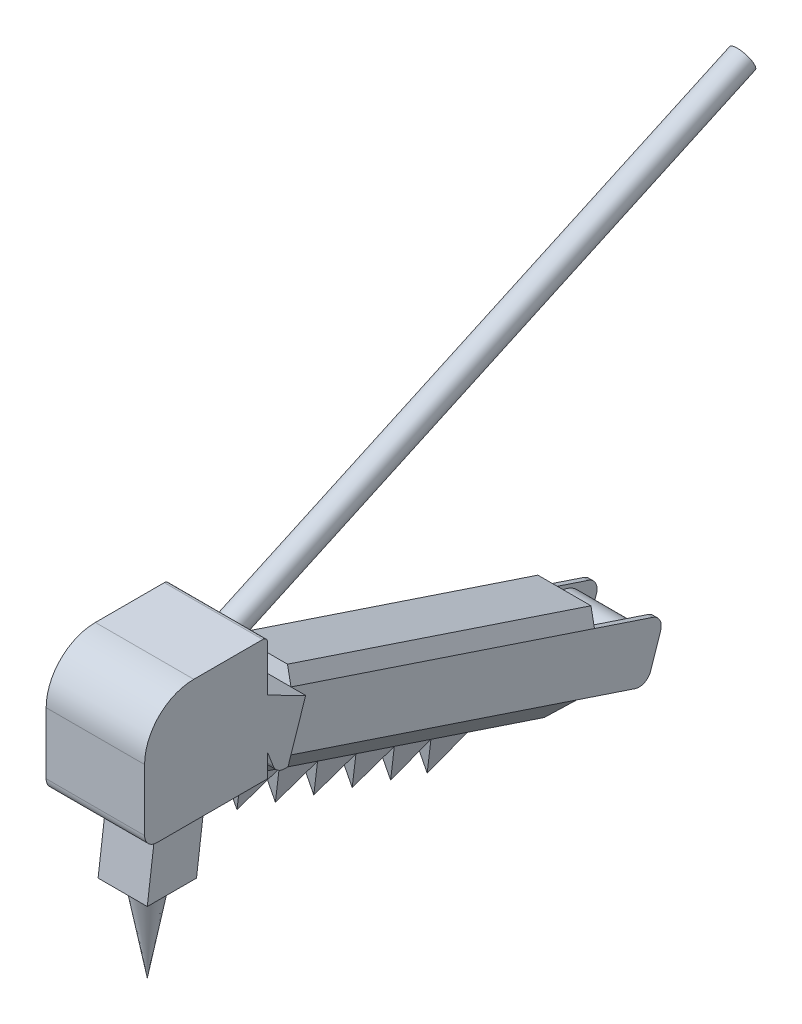
SolidWorks part; units mm, degrees
ref_plane "Front Plane" through (0, 0, 0) normal (0, 0, 1) x (1, 0, 0)
ref_plane "Top Plane" through (0, 0, 0) normal (0, 1, 0) x (1, 0, 0)
ref_plane "Right Plane" through (0, 0, 0) normal (1, 0, 0) x (0, 0, -1)
other "Configuration Table"
sketch "Sketch2" plane through (0, 0, 0) normal (1, 0, 0) x (0, 0, -1)
  line L8 (0, 0) -> (0, 50)
  line L9 (0, 50) -> (50, 50)
  line L10 (50, 50) -> (50, 29.4102)
  line L16 (50, 0) -> (0, 0)
  line L17 (50, 0) -> (50, 9.232)
  line L22 (50, 9.232) -> (53.5278, 0.0614)
  line L25 (65.4524, 21.5893) -> (50, 29.4102)
  line L26 (53.5278, 0.0614) -> (58.2765, 0.0614)
  line L27 (65.4524, 21.5893) -> (58.2765, 0.0614)
  dimension "D1" = 50
  dimension "D2" = 50
  dimension "D3" = 50
extrude "Boss-Extrude1" add sketch "Sketch2" along normal blind 40
fillet "Fillet1" radius 20 1 edges at (20, 50, 0)
fillet "Fillet2" radius 5 1 edges at (20, 0, 0)
ref_plane "Plane1" through (20, 0, 0) normal (1, 0, 0) x (0, 0, -1)
sketch "Sketch4" plane through (20, 0, 0) normal (1, 0, 0) x (0, 0, -1)
  line L0 (25, 6.5797) -> (25, -21.4147) construction
  line L1 (15, 0) -> (11.0974, -30.529)
  line L2 (5, 0) -> (50, 0) construction
  line L3 (11.0974, -30.529) -> (31.0974, -30.529)
  line L4 (31.0974, -30.529) -> (35, 0)
  line L5 (0, 30) -> (0, 5) construction
  line L6 (50, 0) -> (50, 9.232) construction
  line L7 (15, 0) -> (35, 0)
  dimension "D1" = 15
  dimension "D2" = 15
  dimension "D3" = 10
extrude "Boss-Extrude2" add sketch "Sketch4" along normal mid plane 20
sketch "Sketch5" plane through (20, 0, 0) normal (1, 0, 0) x (0, 0, -1)
  line L0 (21.0974, -30.529) -> (21.0974, -46.9338) construction
  line L1 (11.0974, -30.529) -> (31.0974, -30.529) construction
  line L2 (21.0974, -30.529) -> (27.6649, -30.529)
  line L3 (27.6649, -30.529) -> (21.0974, -65.6782)
  line L4 (21.0974, -30.529) -> (21.0974, -65.6782)
revolve "Revolve1" add sketch "Sketch5" angle 360 about L0
fillet "Fillet3" radius 5 1 edges at (20, 0.0614, -53.5278)
fillet "Fillet4" radius 2 1 edges at (20, 50, -50)
sketch "Sketch7" plane through (0, -17.4768, -52.4304) normal (0, -0.3162, -0.9487) x (-1, 0, 0)
  line L1 (-5.963, 18.4869) -> (-16, 8.3482)
  line L2 (-34.037, 18.4869) -> (-24, 8.3482)
  line L5 (-24, 8.3482) -> (-16, 8.3482)
  line L7 (-20, 5.9318) -> (-20, 79.4839) construction
  line L9 (-20, -19.1285) -> (-20, 3.5593) construction
  line L10 (-40, 18.4869) -> (0, 18.4869) construction
  line L11 (-30, -19.1285) -> (-10, -19.1285) construction
  line L12 (-20, 56.453) -> (-20, -56.453) construction
  line L13 (-34.037, 46.9552) -> (-5.963, 46.9552)
  line L14 (-5.963, 46.9552) -> (-5.963, 18.4869)
  line L16 (-30, 11.068) -> (-10, 11.068) construction
  line L18 (-34.037, 46.9552) -> (-34.037, 18.4869)
  line L19 (-20, 11.068) -> (-20, 5.9318)
  point P15 (-20, 46.9552)
  dimension "D1" = 8
extrude "Boss-Extrude6" add sketch "Sketch7" along normal blind 100
sketch "Sketch10" plane through (20, 0, 0) normal (1, 0, 0) x (0, 0, -1)
  line L2 (149.9387, -41.1798) -> (55.0704, -9.557) construction
  line L15 (149.9387, -41.1798) -> (55.0704, -9.557) construction
  line L16 (55.0704, -9.557) -> (149.9387, -41.1798)
  line L30 (153.1448, -31.5614) -> (149.9387, -41.1798) construction
  line L31 (55.0704, -9.557) -> (57.5485, -24.6711)
  line L32 (57.5485, -24.6711) -> (70.6752, -14.7586)
  line L33 (70.6752, -14.7586) -> (73.1534, -29.8728)
  line L34 (73.1534, -29.8728) -> (86.2801, -19.9603)
  line L35 (86.2801, -19.9603) -> (88.7583, -35.0744)
  line L36 (88.7583, -35.0744) -> (101.885, -25.1619)
  line L37 (101.885, -25.1619) -> (104.3631, -40.276)
  line L38 (104.3631, -40.276) -> (117.4899, -30.3635)
  line L39 (117.4899, -30.3635) -> (119.968, -45.4777)
  line L40 (119.968, -45.4777) -> (132.3587, -35.3198)
  line L41 (132.3587, -35.3198) -> (134.8368, -50.4339)
  line L42 (134.8368, -50.4339) -> (147.2274, -40.276)
extrude "Boss-Extrude8" add sketch "Sketch10" along normal mid plane 8
sketch "Sketch20" plane through (0, -49.0996, -147.2987) normal (0, -0.3162, -0.9487) x (-1, 0, 0)
  line L10 (-34.037, 41.1842) -> (-30.7805, 46.9552)
  line L11 (-20, 56.453) -> (-20, -56.453) construction
  line L12 (-5.963, 41.1842) -> (-9.2195, 46.9552)
  line L13 (-30.7805, 46.9552) -> (-34.037, 46.9552)
  line L14 (-34.037, 46.9552) -> (-34.037, 18.4869) construction
  line L16 (-5.963, 18.4869) -> (-5.963, 46.9552)
  line L17 (-5.963, 46.9552) -> (-34.037, 46.9552)
  line L18 (-34.037, 46.9552) -> (-34.037, 18.4869)
  line L19 (-34.037, 18.4869) -> (-24, 8.3482)
  line L20 (-24, 8.3482) -> (-16, 8.3482)
  line L21 (-16, 8.3482) -> (-5.963, 18.4869)
  line L22 (-5.963, 41.1842) -> (-5.963, 46.9552)
  line L23 (-5.963, 46.9552) -> (-9.2195, 46.9552)
  line L24 (-34.037, 46.9552) -> (-34.037, 41.1842)
  dimension "D1" = 0
sketch "Sketch23" plane through (0, -49.0996, -147.2987) normal (0, -0.3162, -0.9487) x (-1, 0, 0)
  line L0 (-20, -5.2141) -> (-16, -5.2067)
  line L1 (-16, -5.2067) -> (-16, 8.3482) construction
  line L2 (-16, -5.2067) -> (-16, 8.3482)
  line L3 (-16, 8.3482) -> (-20, -5.2141)
  line L4 (-24, 8.3482) -> (-20, -5.2141)
  line L5 (-24, -5.2067) -> (-24, 8.3482)
  line L6 (-24, -5.2067) -> (-24, 8.3482) construction
  line L7 (-24, -5.2067) -> (-20, -5.2141)
extrude "Cut-Extrude5" cut sketch "Sketch23" against normal blind 102 contours L2 L3 L0 | L5 L7 L4
sketch "Sketch24" plane through (0, -49.0996, -147.2987) normal (0, -0.3162, -0.9487) x (-1, 0, 0)
  line L6 (-5.963, 18.4869) -> (-5.963, 46.9552)
  line L7 (-5.963, 46.9552) -> (-34.037, 46.9552)
  line L8 (-34.037, 46.9552) -> (-34.037, 18.4869)
  line L9 (-34.037, 18.4869) -> (-24, 8.3482)
  line L10 (-24, 8.3482) -> (-16, 8.3482)
  line L11 (-16, 8.3482) -> (-5.963, 18.4869)
  line L12 (-5.963, 18.4869) -> (-5.963, 46.9552)
  line L13 (-5.963, 46.9552) -> (-34.037, 46.9552)
  line L14 (-34.037, 46.9552) -> (-34.037, 18.4869)
  line L15 (-34.037, 18.4869) -> (-24, 8.3482)
  line L16 (-24, 8.3482) -> (-16, 8.3482)
  line L17 (-16, 8.3482) -> (-5.963, 18.4869)
  dimension "D1" = 0
extrude "Boss-Extrude14" add sketch "Sketch24" along normal blind 30
extrude "Cut-Extrude4" cut sketch "Sketch20" against normal mid plane 200
sketch "Sketch25" plane through (0, -58.5864, -175.7592) normal (0, -0.3162, -0.9487) x (-1, 0, 0)
  line L1 (-34.037, 41.1792) -> (-32.037, 41.1792)
  line L2 (-34.037, 41.1792) -> (-34.037, 18.4869)
  line L3 (-34.037, 18.4869) -> (-32.037, 18.4869)
  line L4 (-32.037, 41.1792) -> (-32.037, 18.4869)
  line L5 (-5.963, 41.1842) -> (-7.963, 41.1842)
  line L6 (-5.963, 41.1842) -> (-5.963, 18.4869)
  line L7 (-5.963, 18.4869) -> (-7.963, 18.4869)
  line L8 (-7.963, 41.1842) -> (-7.963, 18.4869)
  dimension "D1" = 2
  dimension "D2" = 2
extrude "Boss-Extrude15" add sketch "Sketch25" along normal blind 30
sketch "Sketch26" plane through (34.037, 0, 0) normal (1, 0, 0) x (0, 0, -1)
  circle A2 centre (200.7211, -35.4576) radius 10
  dimension "D1" = 20
extrude "Boss-Extrude16" add sketch "Sketch26" against normal up to surface (26.074 mm away) up to face at (7.963, -35.0253, -199.4243)
fillet "Fillet5" radius 5 4 edges at (6.963, -29.0025, -217.2433) (6.963, -50.5351, -210.0658) (33.037, -50.5351, -210.0658) (33.037, -29.0072, -217.2418)
sketch "Sketch28" plane through (20, 0, 0) normal (1, 0, 0) x (0, 0, -1)
  line L0 (50, 33.7696) -> (50, 39.2717)
  line L1 (50, 29.4102) -> (50, 48) construction
  line L2 (50, 39.2717) -> (262.9817, 137.0797)
  line L3 (262.9817, 137.0797) -> (265.0684, 132.536)
  line L4 (265.0684, 132.536) -> (50, 33.7696)
  dimension "D1" = 5
revolve "Revolve3" add sketch "Sketch28" angle 360 about L2
